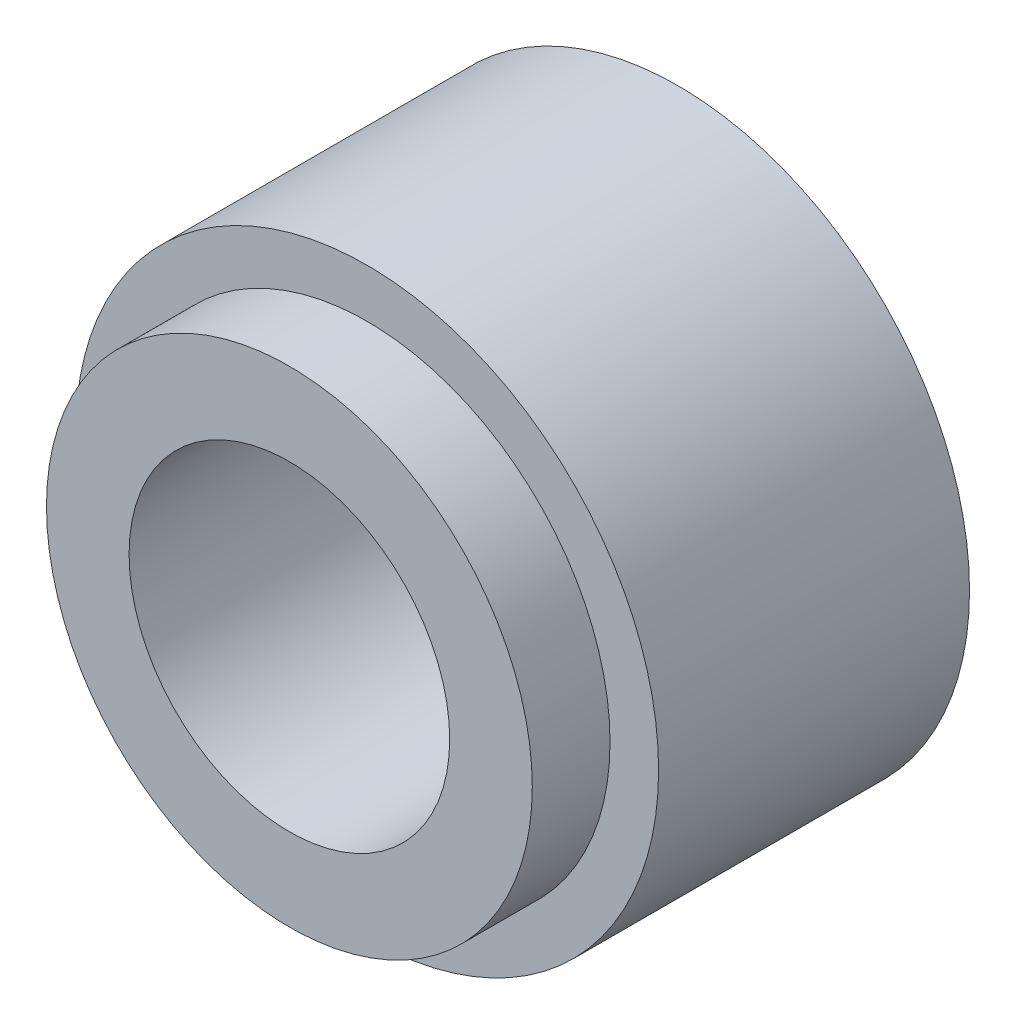
SolidWorks part; units mm, degrees
material "Q235B"
ref_plane "Front Plane" through (0, 0, 0) normal (0, 0, 1) x (1, 0, 0)
ref_plane "Top Plane" through (0, 0, 0) normal (0, 1, 0) x (1, 0, 0)
ref_plane "Right Plane" through (0, 0, 0) normal (1, 0, 0) x (0, 0, -1)
sketch "Sketch1" plane through (0, 0, 0) normal (0, 1, 0) x (1, 0, 0)
  line L0 (0, 0) -> (0, 20) construction
  line L1 (7.5, 0) -> (12.5, 0)
  line L2 (12.5, 0) -> (12.5, 4)
  line L3 (12.5, 4) -> (15, 4)
  line L4 (15, 4) -> (15, 20)
  line L5 (15, 20) -> (7.5, 20)
  line L6 (7.5, 20) -> (7.5, 0)
  dimension "D1" = 15
  dimension "D2" = 25
  dimension "D3" = 20
  dimension "D4" = 16
  dimension "D5" = 30
revolve "Revolve1" add sketch "Sketch1" angle 360 about L0
hole_wizard "M18x1.5 Tapped Hole1" positions "Sketch2" profile "Sketch3" tap size "M18x1.5" standard "GB"
sketch "Sketch2" plane through (0, 0, -20) normal (0, 0, -1) x (-1, 0, 0)
  point P0 (0, 0)
sketch "Sketch3" plane through (0, 0, -20) normal (1, 0, 0) x (0, 1, 0)
  line L0 (0, 0) -> (0, 48.4571)
  line L1 (0, 48.4571) -> (8.25, 43.5)
  line L2 (8.25, 43.5) -> (8.25, 0)
  line L5 (8.25, 0) -> (0, 0)
  line L10 (0, 48.4571) -> (-8.25, 43.5) construction
  line L11 (0, -6.35) -> (0, 107.95) construction
  dimension "螺纹孔钻头直径" = 16.5
  dimension "螺纹孔钻头深度" = 43.5
  dimension "导头角度" = 118
cosmetic thread "Hole thread 1"
chamfer "Chamfer1" distance 0.75 angle 45 1 edges at (-8.25, 0, -20)
